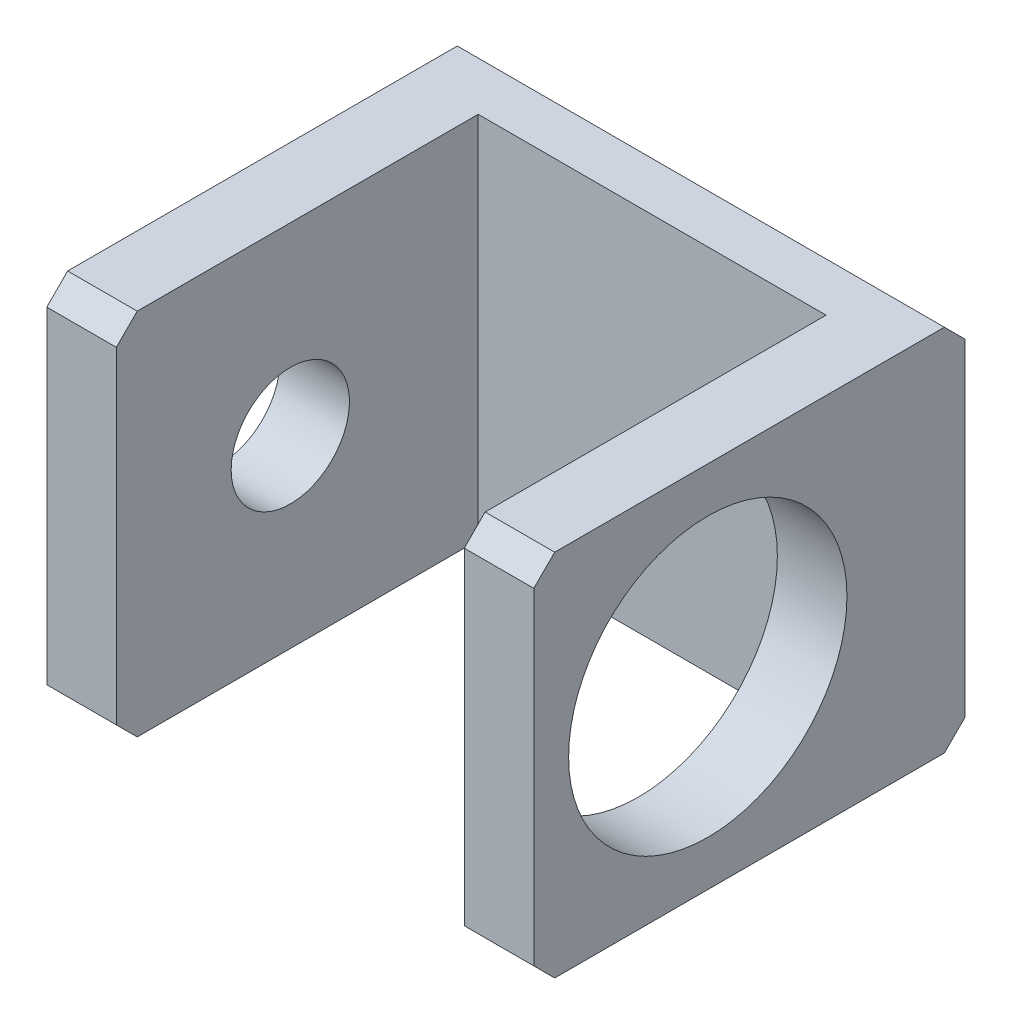
from build123d import *

# Parameters (mm, degrees)
EXTRUDE_1_DEPTH     = 26.5
CUT_EXTRUDE_2_REACH = 99.192
SKETCH_7_R          = 8.5
CUT_EXTRUDE_3_REACH = 92.257
SKETCH_8_R          = 20
CHAMFER_2_SIZE      = 3
CHAMFER_3_SIZE      = 3


with BuildPart() as part:
    # 草图1 → 凸台-拉伸1 (new, symmetric)
    with BuildSketch(Plane(origin=(0, 0, 0), x_dir=(1, 0, 0), z_dir=(0, 1, 0))):
        Polygon((0, 0), (0, 52), (50, 52), (50, 0), (60, 0), (60, 62), (-10, 62), (-10, 0), align=None)
    extrude(amount=EXTRUDE_1_DEPTH, both=True)

    # 草图7 → 切除-拉伸2 (cut, up to next)
    with BuildSketch(Plane.ZY.offset(10), mode=Mode.PRIVATE) as cut_extrude_2_sk1:
        with Locations((-25, 0)):
            Circle(SKETCH_7_R)
    cut_extrude_2_tool1 = extrude(cut_extrude_2_sk1.sketch, amount=-CUT_EXTRUDE_2_REACH, mode=Mode.PRIVATE) & part.part
    add(cut_extrude_2_tool1.solids().sort_by_distance((-10, 0, -25))[0], mode=Mode.SUBTRACT)

    # 草图8 → 切除-拉伸3 (cut, up to next)
    with BuildSketch(Plane.ZY.offset(-50), mode=Mode.PRIVATE) as cut_extrude_3_sk1:
        with Locations((-25, 0)):
            Circle(SKETCH_8_R)
    cut_extrude_3_tool1 = extrude(cut_extrude_3_sk1.sketch, amount=-CUT_EXTRUDE_3_REACH, mode=Mode.PRIVATE) & part.part
    add(cut_extrude_3_tool1.solids().sort_by_distance((50, 0, -25))[0], mode=Mode.SUBTRACT)

    # 倒角2
    chamfer_2_edges = [part.edges().sort_by_distance(p)[0] for p in [
        (25, 26.5, -62),
        (25, -26.5, -62),
    ]]
    chamfer(chamfer_2_edges, length=CHAMFER_2_SIZE)

    # 倒角3
    chamfer_3_edges = [part.edges().sort_by_distance(p)[0] for p in [
        (-5, -26.5, 0),
        (55, 26.5, 0),
        (-5, 26.5, 0),
        (55, -26.5, 0),
    ]]
    chamfer(chamfer_3_edges, length=CHAMFER_3_SIZE)


solid = part.part
